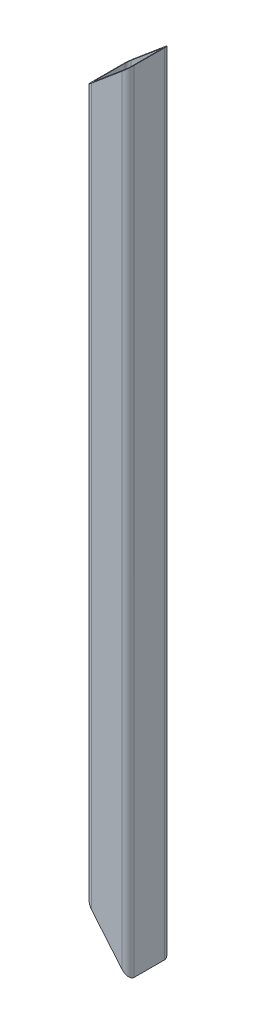
from build123d import *

# Parameters (mm, degrees)
F_19_WELDMEMBERFEAT_4_MORE_IN_5_FILES_DEPTH = 1302
CUT_EXTRUDE1_DEPTH                          = 1305.350029708
CUT_EXTRUDE1_DEPTH_BACK                     = 1305.350029708


with BuildPart() as part:
    # Sketch1 → 19 (WeldMemberFeat) (+4 more in 5 files) Cold-formed hollow square steel (GB/T 6728-2002) 70×70×5(1) (new body)
    with BuildSketch(Plane(origin=(0, 0, 0), x_dir=(-1, 0, 0), z_dir=(0, 1, 0))):
        with BuildLine():
            Line((-25, -35), (25, -35))
            ThreePointArc((25, -35), (32.071067812, -32.071067812), (35, -25))
            Line((35, -25), (35, 25))
            ThreePointArc((35, 25), (32.071067812, 32.071067812), (25, 35))
            Line((25, 35), (-25, 35))
            ThreePointArc((-25, 35), (-32.071067812, 32.071067812), (-35, 25))
            Line((-35, 25), (-35, -25))
            ThreePointArc((-35, -25), (-32.071067812, -32.071067812), (-25, -35))
        make_face()
        with BuildLine():
            Line((-25, -30), (25, -30))
            ThreePointArc((25, -30), (28.535533906, -28.535533906), (30, -25))
            Line((30, -25), (30, 25))
            ThreePointArc((30, 25), (28.535533906, 28.535533906), (25, 30))
            Line((25, 30), (-25, 30))
            ThreePointArc((-25, 30), (-28.535533906, 28.535533906), (-30, 25))
            Line((-30, 25), (-30, -25))
            ThreePointArc((-30, -25), (-28.535533906, -28.535533906), (-25, -30))
        make_face(mode=Mode.SUBTRACT)
    extrude(amount=F_19_WELDMEMBERFEAT_4_MORE_IN_5_FILES_DEPTH)

    # Sketch2 → Cut-Extrude1 (cut, two sides: drawn at the far end of the back side and taken through both)
    with BuildSketch(Plane.XY.offset(35).offset(-CUT_EXTRUDE1_DEPTH_BACK)):
        Polygon((35, 1302), (-35, 1243.247002398), (-35, 1302), align=None)
        Polygon((-35, 83.4), (35, 0), (-35, 0), align=None)
    extrude(amount=CUT_EXTRUDE1_DEPTH + CUT_EXTRUDE1_DEPTH_BACK, mode=Mode.SUBTRACT)


solid = part.part
